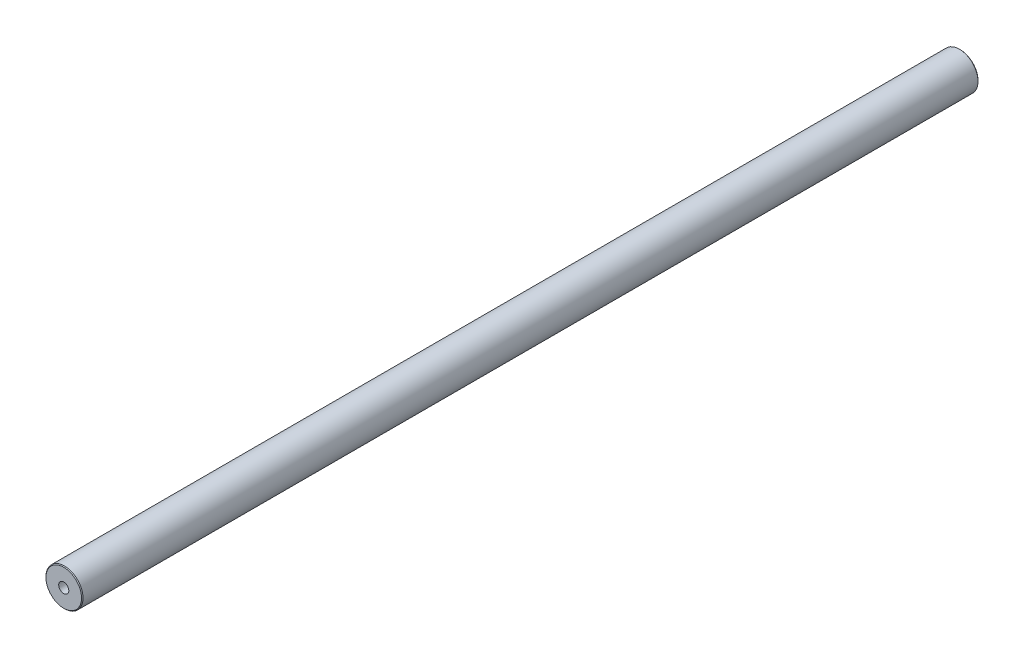
SolidWorks part; units mm, degrees
material "Q235A"
ref_plane "前视基准面" through (0, 0, 0) normal (0, 0, 1) x (1, 0, 0)
ref_plane "上视基准面" through (0, 0, 0) normal (0, 1, 0) x (1, 0, 0)
ref_plane "右视基准面" through (0, 0, 0) normal (1, 0, 0) x (0, 0, -1)
sketch "草图1" plane through (0, 0, 0) normal (0, 0, 1) x (1, 0, 0)
  circle A0 centre (0, 0) radius 12.5
  dimension "D1" = 25
extrude "凸台-拉伸1" add sketch "草图1" along normal blind 605
hole_wizard "M8 螺纹孔1" positions "草图2" profile "草图4" tap size "M8" standard "GB"
sketch "草图2" plane through (0, 0, 0) normal (0, 0, 1) x (1, 0, 0)
  point P0 (0, 0)
sketch "草图4" plane through (0, 0, 0) normal (1, 0, 0) x (0, 1, 0)
  line L0 (0, 0) -> (0, 24.2929)
  line L1 (0, 24.2929) -> (3.4, 22.25)
  line L2 (3.4, 22.25) -> (3.4, 0)
  line L5 (3.4, 0) -> (0, 0)
  line L10 (0, 24.2929) -> (-3.4, 22.25) construction
  line L11 (0, -6.35) -> (0, 107.95) construction
  dimension "螺纹孔钻头直径" = 6.8
  dimension "螺纹孔钻头深度" = 22.25
  dimension "导头角度" = 118
cosmetic thread "孔螺蚊线1"
chamfer "倒角1" distance 0.5 angle 45 2 edges at (12.5, 0, 605) (12.5, 0, 0)
hole_wizard "M8 螺纹孔2" positions "草图5" profile "草图6" tap size "M8" standard "GB"
sketch "草图5" plane through (0, 0, 605) normal (0, 0, 1) x (1, 0, 0)
  point P0 (0, 0)
sketch "草图6" plane through (0, 0, 605) normal (1, 0, 0) x (0, -1, 0)
  line L0 (0, 0) -> (0, 21.7929)
  line L1 (0, 21.7929) -> (3.4, 19.75)
  line L2 (3.4, 19.75) -> (3.4, 0)
  line L5 (3.4, 0) -> (0, 0)
  line L10 (0, 21.7929) -> (-3.4, 19.75) construction
  line L11 (0, -6.35) -> (0, 107.95) construction
  dimension "螺纹孔钻头直径" = 6.8
  dimension "螺纹孔钻头深度" = 19.75
  dimension "导头角度" = 118
cosmetic thread "孔螺蚊线2"
